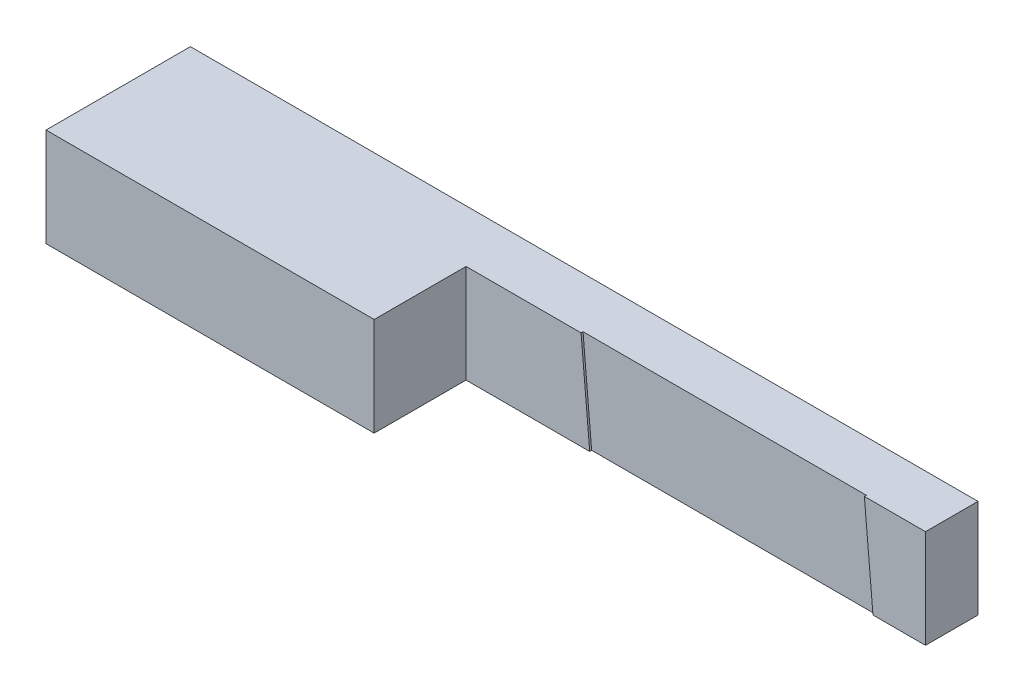
SolidWorks part; units mm, degrees
ref_plane "前视基准面" through (0, 0, 0) normal (0, 0, 1) x (1, 0, 0)
ref_plane "上视基准面" through (0, 0, 0) normal (0, 1, 0) x (1, 0, 0)
ref_plane "右视基准面" through (0, 0, 0) normal (1, 0, 0) x (0, 0, -1)
sketch "草图1" plane through (0, 0, 0) normal (0, 0, 1) x (1, 0, 0)
  line L1 (-60, -7.5) -> (60, -7.5)
  line L2 (-60, -7.5) -> (-60, 7.5)
  line L3 (-60, 7.5) -> (60, 7.5)
  line L4 (60, -7.5) -> (60, 7.5)
  line L5 (-60, -7.5) -> (60, 7.5) construction
  line L6 (-60, 7.5) -> (60, -7.5) construction
  point P0 (0, 0)
  dimension "D1" = 15
  dimension "D2" = 120
extrude "凸台-拉伸1" add sketch "草图1" along normal blind 8
sketch "草图2" plane through (0, 0, 8) normal (0, 0, 1) x (1, 0, 0)
  line L0 (50.6877, 7.5) -> (52, -7.5)
  line L1 (60, 7.5) -> (-60, 7.5) construction
  line L2 (-60, -7.5) -> (60, -7.5) construction
  line L3 (7.5234, 7.5) -> (8.8357, -7.5)
  line L4 (60, -7.5) -> (60, 7.5) construction
  line L5 (7.5234, 7.5) -> (50.6877, 7.5)
  line L6 (8.8357, -7.5) -> (52, -7.5)
  dimension "D1" = 5
  dimension "D2" = 8
  dimension "D3" = 43
extrude "切除-拉伸1" cut sketch "草图2" against normal blind 0.3
sketch "草图3" plane through (0, -7.5, 0) normal (0, -1, 0) x (1, 0, 0)
  line L0 (-60, 0) -> (60, 0) construction
  line L1 (-22, 15) -> (22, 15)
  line L2 (-22, 15) -> (-22, 0)
  line L3 (-22, 0) -> (22, 0)
  line L4 (22, 15) -> (22, 0)
  line L5 (-22, 15) -> (22, 0) construction
  line L6 (-22, 0) -> (22, 15) construction
  point P0 (0, 7.5)
  point P7 (0, 0)
  point P8 (0, 0)
  point P9 (0, 0)
  dimension "D1" = 44
  dimension "D2" = 15
extrude "切除-拉伸2" [suppressed] cut sketch "草图3" against normal blind 1.5
sketch "草图4" [suppressed] plane through (0, -7.5, 0) normal (0, -1, 0) x (1, 0, 0)
  line L0 (-22, 15) -> (-22, 16)
  line L1 (-16, 16) -> (-16, 15)
  line L2 (22, 15) -> (-22, 15) construction
  line L3 (-16, 15) -> (-22, 15)
  line L4 (0, 0) -> (0, 15) construction
  line L5 (22, 15) -> (-22, 15) construction
  line L6 (16, 15) -> (22, 15)
  line L7 (16, 16) -> (16, 15)
  line L8 (22, 15) -> (22, 16)
  arc A0 (-22, 16) -> (-16, 16) centre (-19, 16) cw
  arc A1 (22, 16) -> (16, 16) centre (19, 16) ccw
  dimension "D1" = 3
  dimension "D2" = 1
extrude "切除-拉伸3" [suppressed] cut sketch "草图4" against normal blind 1.5
sketch "草图6" plane through (0, -7.5, 0) normal (0, -1, 0) x (1, 0, 0)
  line L1 (-60, 8) -> (-10, 8)
  line L2 (-60, 8) -> (-60, 22)
  line L3 (-60, 22) -> (-10, 22)
  line L4 (-10, 8) -> (-10, 22)
  dimension "D1" = 50
  dimension "D2" = 14
extrude "凸台-拉伸2" add sketch "草图6" against normal up to surface (15 mm away) up to face at (14.5528, 7.5, 5.925)
